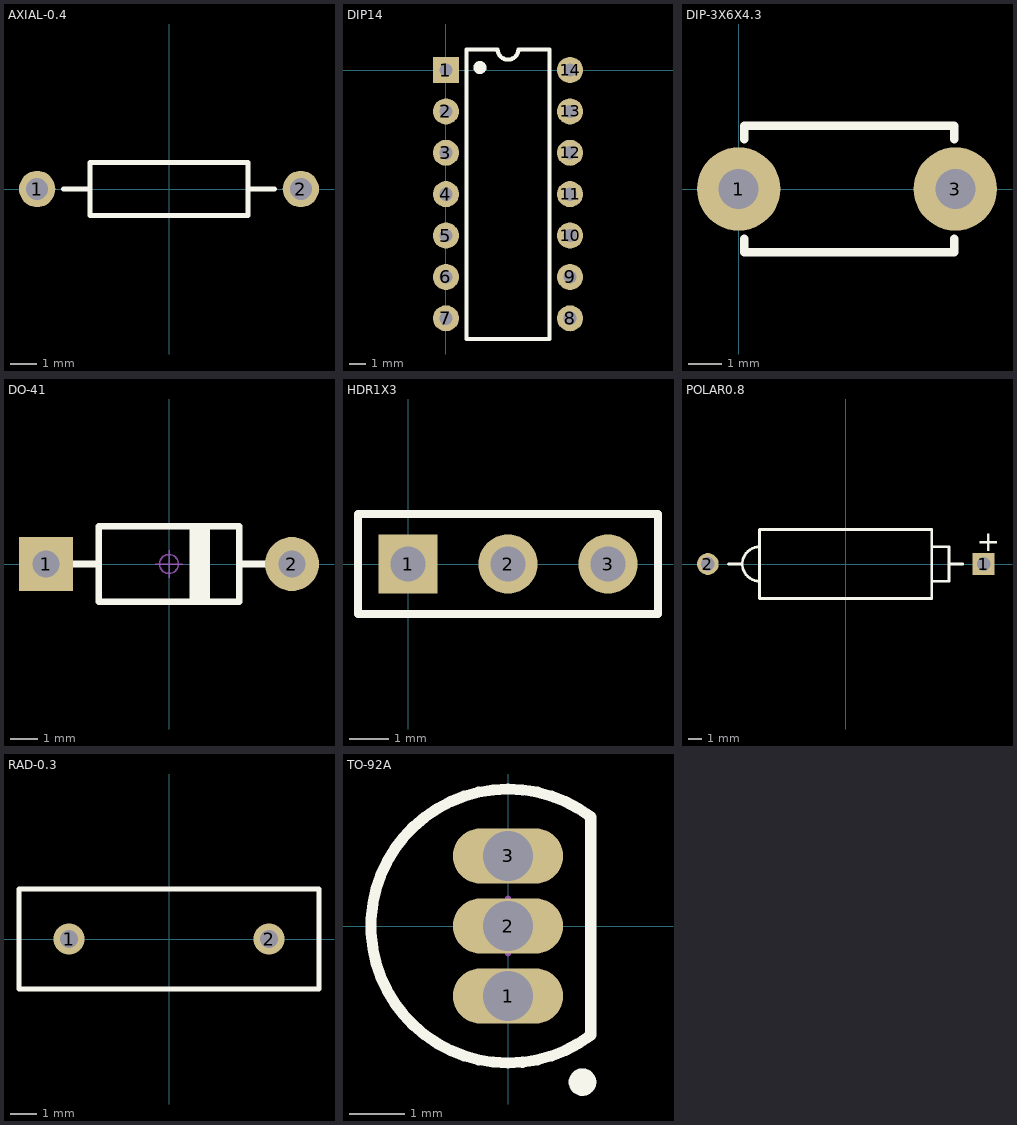
[diagram p0: the footprints below, top view; thin cyan lines are the x and y axes]
# Altium footprint library MISC80621.PcbLib: 8 footprints
Each footprint in its own frame and in the unit in brackets; x right, y up, seen from the top. Pads: shape width x height; smd on the part's side, far side on the other; paste and mask are expansions set on the pad; w line width, h text height; cw(c..) or ccw(c..) is an arc to the next point about the centre after c.

## AXIAL-0.4 [mm] "Axial Device, Thru-Hole; 2 Leads; 0.4 in Pin Spacing"
height 2.032
pads (2):
  round 1.4 hole 0.85: 1(-5.08,0) 2(5.08,0)
Top Overlay:
  lines w0.2: -4.064,0 -3.048,0 ; 3.048,0 4.064,0 ; -3.048,-1.016 3.048,-1.016 3.048,1.016 -3.048,1.016 -3.048,-1.016

## DIP14 [mm]
height 4.58
pads (14):
  rect 1.6x1.6 hole 0.813: 1(0,0)
  round 1.6 hole 0.813: 2(0,-2.54) 3(0,-5.08) 4(0,-7.62) 5(0,-10.16) 6(0,-12.7) 7(0,-15.24) 8(7.62,-15.24) 9(7.62,-12.7) 10(7.62,-10.16) 11(7.62,-7.62) 12(7.62,-5.08) 13(7.62,-2.54) 14(7.62,0)
Top Overlay:
  circle w0.5: c2.085,0.155 r0.15
  lines w0.254: 1.27,-16.51 1.27,1.27 3.175,1.27 ccw(c3.81,1.27) 4.445,1.27 6.35,1.27 6.35,-16.51 1.27,-16.51
3D body "DIP14.STEP": height 5.1, standoff -3.3, extent -0.25,-17.62 7.62,2.38

## DIP-3X6X4.3 [mm]
height 4.58
pads (2):
  round 2.5 hole 1.2: 1(0,0) 3(6.5,0)
Top Overlay:
  lines w0.254: 0.162,-1.499 0.162,-1.9 6.462,-1.9 6.462,-1.499 ; 0.162,1.499 0.162,1.9 6.462,1.9 6.462,1.499
3D body "DIP-3X6X4.3.STEP": height 4.31, standoff -3.49, extent -0.635,-1.75 7.194,1.75

## DO-41 [mm] "2.6*9.1mm (diameter, lead pitch)"
height 2.4
pads (2):
  rect 2x2 hole 1: 1(-4.55,0)
  round 2 hole 1: 2(4.55,0)
Top Overlay:
  rectangle: 0.762,-1.397 1.524,1.397
  lines w0.254: -3.556,0 -2.6,0 ; 2.6,0 3.556,0 ; -2.6,-1.397 2.6,-1.397 2.6,1.397 -2.6,1.397 -2.6,-1.397
Mechanical 15:
  circle w0.05: c0,0 r0.35
  lines w0.05: -0.5,0 0.5,0 ; 0,-0.5 0,0.5
3D body "DO-41.STEP": height 2.65, standoff -3.45, extent -4.925,-1.288 4.975,1.314

## HDR1X3 [mm] "Connector; Header; 3 Position"
height 4.58
pads (3):
  rect 1.5x1.5 hole 0.9: 1(0,0)
  round 1.5 hole 0.9: 2(2.54,0) 3(5.08,0)
Top Overlay:
  lines w0.2: -1.27,-1.27 6.35,-1.27 6.35,1.27 -1.27,1.27 -1.27,-1.27

## POLAR0.8 [mm] "Polarized Capacitor; 2 Leads"
height 5.08
pads (2):
  rect 1.6x1.6 hole 1: 1(10.16,0)
  round 1.6 hole 1: 2(-10.16,0)
Top Overlay:
  lines w0.2: -8.636,0 -7.62,0 ; -6.35,-1.27 cw(c-6.35,0) -6.35,1.27 ; 6.35,-1.27 7.62,-1.27 7.62,1.27 6.35,1.27 ; 7.62,0 8.636,0 ; -6.35,-2.54 -6.35,2.54 6.35,2.54 6.35,-2.54 -6.35,-2.54
  text "+" at 9.652,0.95 h1.5

## RAD-0.3 [mm] "Radial Cap, Thru-Hole; 2 Leads; 0.3 in Pin Spacing"
height 6
pads (2):
  round 1.2 hole 0.7: 1(-3.81,0) 2(3.81,0)
Top Overlay:
  lines w0.2: -5.715,-1.905 5.715,-1.905 5.715,1.905 -5.715,1.905 -5.715,-1.905

## TO-92A [mm] "TO, Flat Index; 3 In-Line, Axial Leads; Body Dia. 4.5mm; Leads 0.51 x 0.48 mm (max)"
height 6.86
pads (3):
  oval 2x1 hole 0.9: 1(0,-1.27) 2(0,0) 3(0,1.27)
Top Overlay:
  circle w0.25: c1.35,-2.83 r0.125
  lines w0.2: 1.5,-1.98 cw(c0,0) 1.5,1.98 1.5,-1.98
Mechanical 13:
  lines w0.1: 1.5,-1.98 cw(c0,0) 1.5,1.98 1.5,-1.98
Mechanical 15:
  lines w0.1: -0.5,0 0.5,0 ; 0,-0.5 0,0.5
3D body: height 6.86, standoff 2.2, extent -2.485,-2.495 1.501,2.495